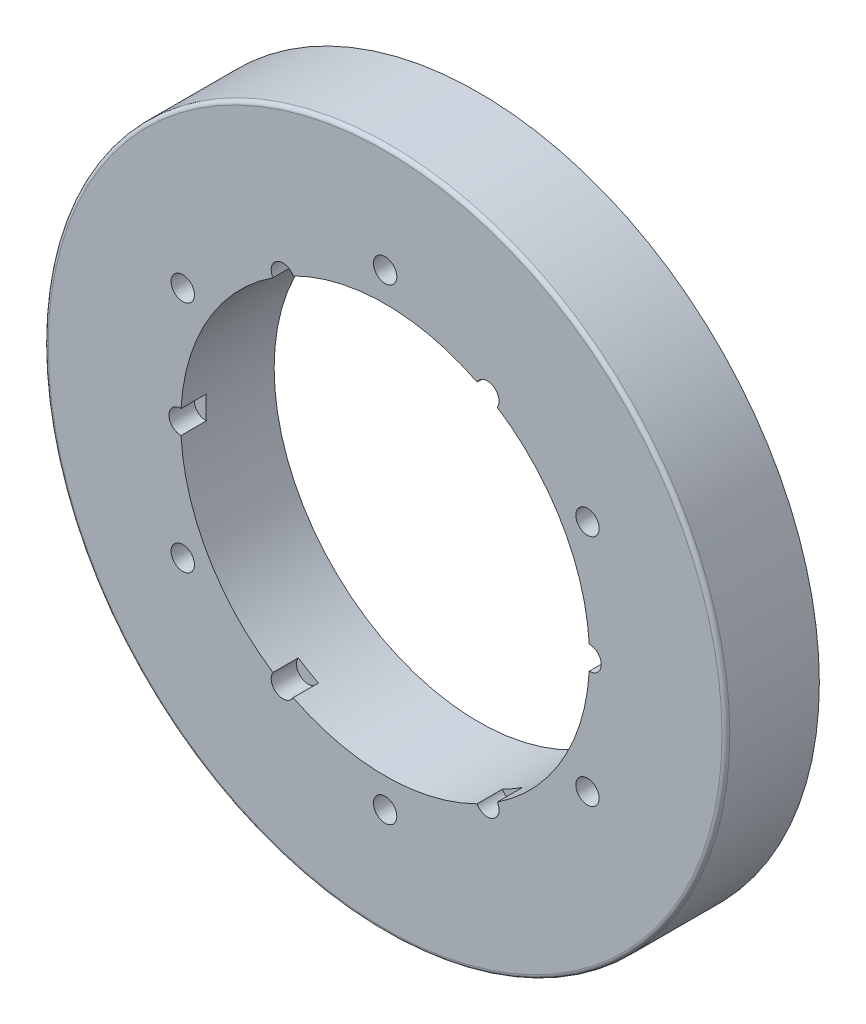
from build123d import *

# Parameters (mm, degrees)
M14_CLEARANCE_HOLE1_D          = 16.4
M14_CLEARANCE_HOLE1_DEPTH      = 28
F_12_0_12_DIAMETER_HOLE1_D     = 12
F_12_0_12_DIAMETER_HOLE1_DEPTH = 13
HOLE1_D                        = 210


with BuildPart() as part:
    # Sketch1 → Revolve1 (revolve)
    with BuildSketch(Plane(origin=(0, 953.248948069, 0), x_dir=(1, 0, 0), z_dir=(0, 1, 0))):
        with BuildLine():
            Line((440.076894512, -691.106692253), (265.076894512, -691.106692253))
            Line((265.076894512, -691.106692253), (265.076894512, -739.106692253))
            Line((265.076894512, -739.106692253), (438.076894512, -739.106692253))
            ThreePointArc((438.076894512, -739.106692253), (439.491108075, -738.520905816), (440.076894512, -737.106692253))
            Line((440.076894512, -737.106692253), (440.076894512, -691.106692253))
        make_face()
    revolve(axis=Axis((265.076894512, 953.248948069, 691.106692253), (0, 0, 1)))

    # M14 Clearance Hole1
    with Locations(Plane(origin=(0, 0, 691.106692253), x_dir=(-1, 0, 0), z_dir=(0, 0, -1))):
        with Locations((-123.048728292, 1035.248948069), (-123.048728292, 871.248948069), (-265.076894512, 789.248948069), (-407.105060733, 871.248948069), (-407.105060733, 1035.248948069), (-265.076894512, 1117.248948069)):
            Hole(M14_CLEARANCE_HOLE1_D / 2, depth=M14_CLEARANCE_HOLE1_DEPTH)

    # Ø12.0 (12) Diameter Hole1
    with Locations(Plane.XY.offset(739.106692253)):
        with Locations((370.076894512, 953.248948069), (317.576894512, 1044.181615466), (160.076894512, 953.248948069), (212.576894512, 862.316280672), (317.576894512, 862.316280672), (212.576894512, 1044.181615466), (265.076894512, 833.248948069), (161.153846058, 893.248948069), (161.153846058, 1013.248948069), (265.076894512, 1073.248948069), (368.999942966, 1013.248948069), (368.999942966, 893.248948069)):
            Hole(F_12_0_12_DIAMETER_HOLE1_D / 2, depth=F_12_0_12_DIAMETER_HOLE1_DEPTH)

    # Hole1 (through all)
    with Locations(Plane(origin=(0, 0, 691.106692253), x_dir=(-1, 0, 0), z_dir=(0, 0, -1))):
        with Locations((-265.076894512, 953.248948069)):
            Hole(HOLE1_D / 2)


solid = part.part
